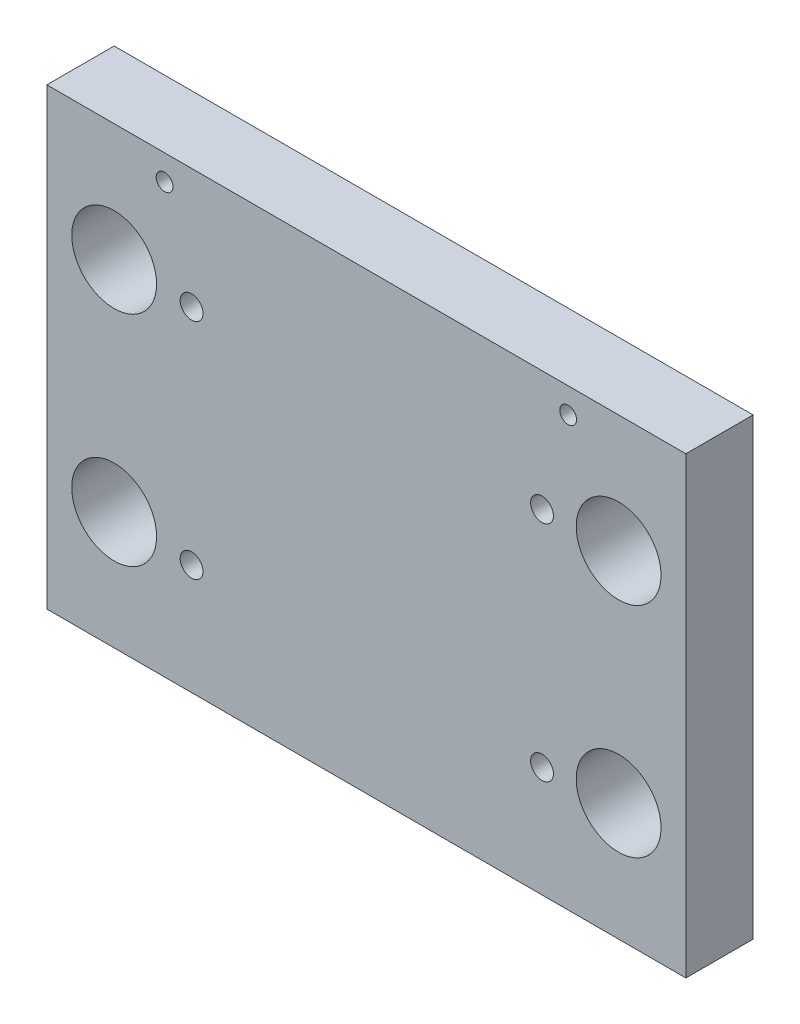
SolidWorks part; units mm, degrees
ref_plane "Front Plane" through (0, 0, 0) normal (0, 0, 1) x (1, 0, 0)
ref_plane "Top Plane" through (0, 0, 0) normal (0, 1, 0) x (1, 0, 0)
ref_plane "Right Plane" through (0, 0, 0) normal (1, 0, 0) x (0, 0, -1)
other "Configuration Table"
sketch "Sketch1" plane through (0, 0, 0) normal (0, 0, 1) x (1, 0, 0)
  line L1 (-95, 67.5) -> (95, 67.5)
  line L2 (-95, 67.5) -> (-95, -67.5)
  line L3 (-95, -67.5) -> (95, -67.5)
  line L4 (95, 67.5) -> (95, -67.5)
  line L5 (-95, 67.5) -> (95, -67.5) construction
  line L6 (-95, -67.5) -> (95, 67.5) construction
  line L11 (-75, 32.5) -> (75, -32.5) construction
  line L12 (-75, -32.5) -> (75, 32.5) construction
  circle A0 centre (-75, 32.5) radius 12.6119
  circle A1 centre (-75, -32.5) radius 12.6119
  circle A2 centre (75, 32.5) radius 12.6119
  circle A3 centre (75, -32.5) radius 12.6119
  point P0 (0, 0)
  point P6 (0, 0)
  dimension "D1" = 32.5
  dimension "D2" = 32.5
  dimension "D3" = 32.5
  dimension "D4" = 32.5
  dimension "D5" = 75
  dimension "D6" = 75
extrude "Boss-Extrude1" add sketch "Sketch1" along normal blind 20
sketch "Sketch21" plane through (0, 0, 0) normal (0, 0, -1) x (-1, 0, 0)
  line L0 (-95, 67.5) -> (95, 67.5) construction
  line L1 (0, 67.5) -> (0, 60)
  line L2 (0, 60) -> (-60, 60)
  line L3 (0, 60) -> (60, 60)
hole_wizard "M6 Tapped Hole6" positions "Sketch24" profile "Sketch23" tap size "M6" standard "GB" end condition through all
sketch "Sketch24" plane through (0, 0, 0) normal (0, 0, -1) x (-1, 0, 0)
  point P0 (-60, 60)
  point P3 (60, 60)
sketch "Sketch23" plane through (60, 60, 0) normal (1, 0, 0) x (0, 1, 0)
  line L0 (0, 0) -> (0, 20)
  line L1 (0, 20) -> (2.5, 20)
  line L2 (2.5, 20) -> (2.5, 0)
  line L5 (2.5, 0) -> (0, 0)
  line L11 (0, -6.35) -> (0, 107.95) construction
  dimension "通孔螺纹孔钻头直径" = 5
  dimension "通孔螺纹孔钻头深度" = 20
cosmetic thread "Cosmetic Thread14" parameters "D2"=6
cosmetic thread "Cosmetic Thread15" parameters "D2"=6
hole_wizard "M8 Tapped Hole1" positions "Sketch27" profile "Sketch26" tap size "M8" standard "GB"
sketch "Sketch27" plane through (0, 0, 20) normal (0, 0, 1) x (1, 0, 0)
  point P0 (-51.9674, 31.8209)
  point P2 (-51.9674, -34.6227)
  point P4 (52.2343, -34.6227)
  point P6 (52.2343, 31.8209)
sketch "Sketch26" plane through (-51.9674, 31.8209, 20) normal (1, 0, 0) x (0, -1, 0)
  line L0 (0, 0) -> (0, 21.7929)
  line L1 (0, 21.7929) -> (3.4, 19.75)
  line L2 (3.4, 19.75) -> (3.4, 0)
  line L5 (3.4, 0) -> (0, 0)
  line L10 (0, 21.7929) -> (-3.4, 19.75) construction
  line L11 (0, -6.35) -> (0, 107.95) construction
  dimension "螺纹孔钻头直径" = 6.8
  dimension "螺纹孔钻头深度" = 19.75
  dimension "导头角度" = 118
cosmetic thread "Cosmetic Thread16" parameters "D1"=16, "D2"=8
cosmetic thread "Cosmetic Thread17" parameters "D1"=16, "D2"=8
cosmetic thread "Cosmetic Thread18" parameters "D1"=16, "D2"=8
cosmetic thread "Cosmetic Thread19" parameters "D1"=16, "D2"=8
